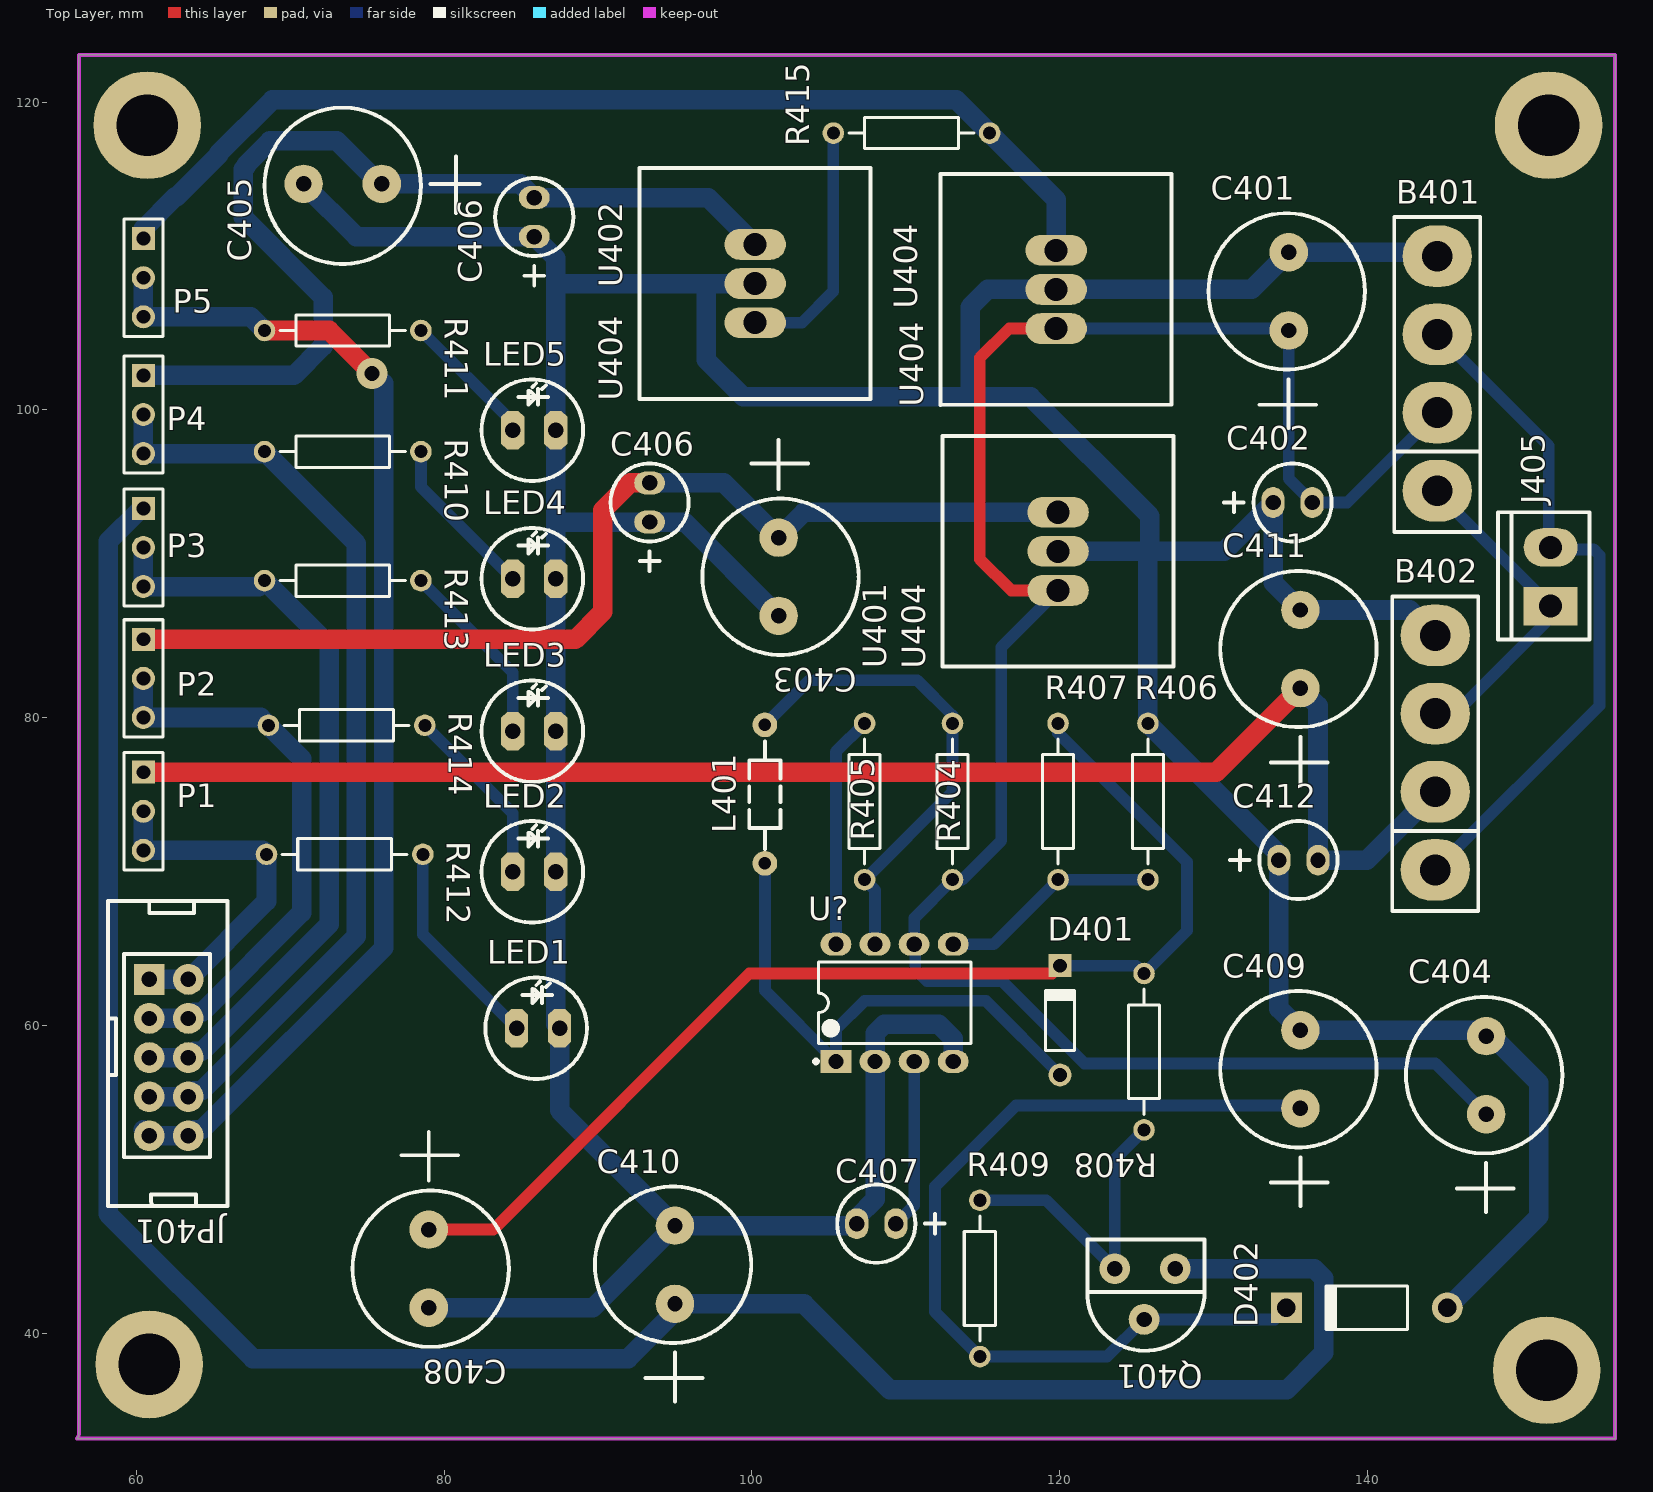
[diagram p0: Top Layer view]
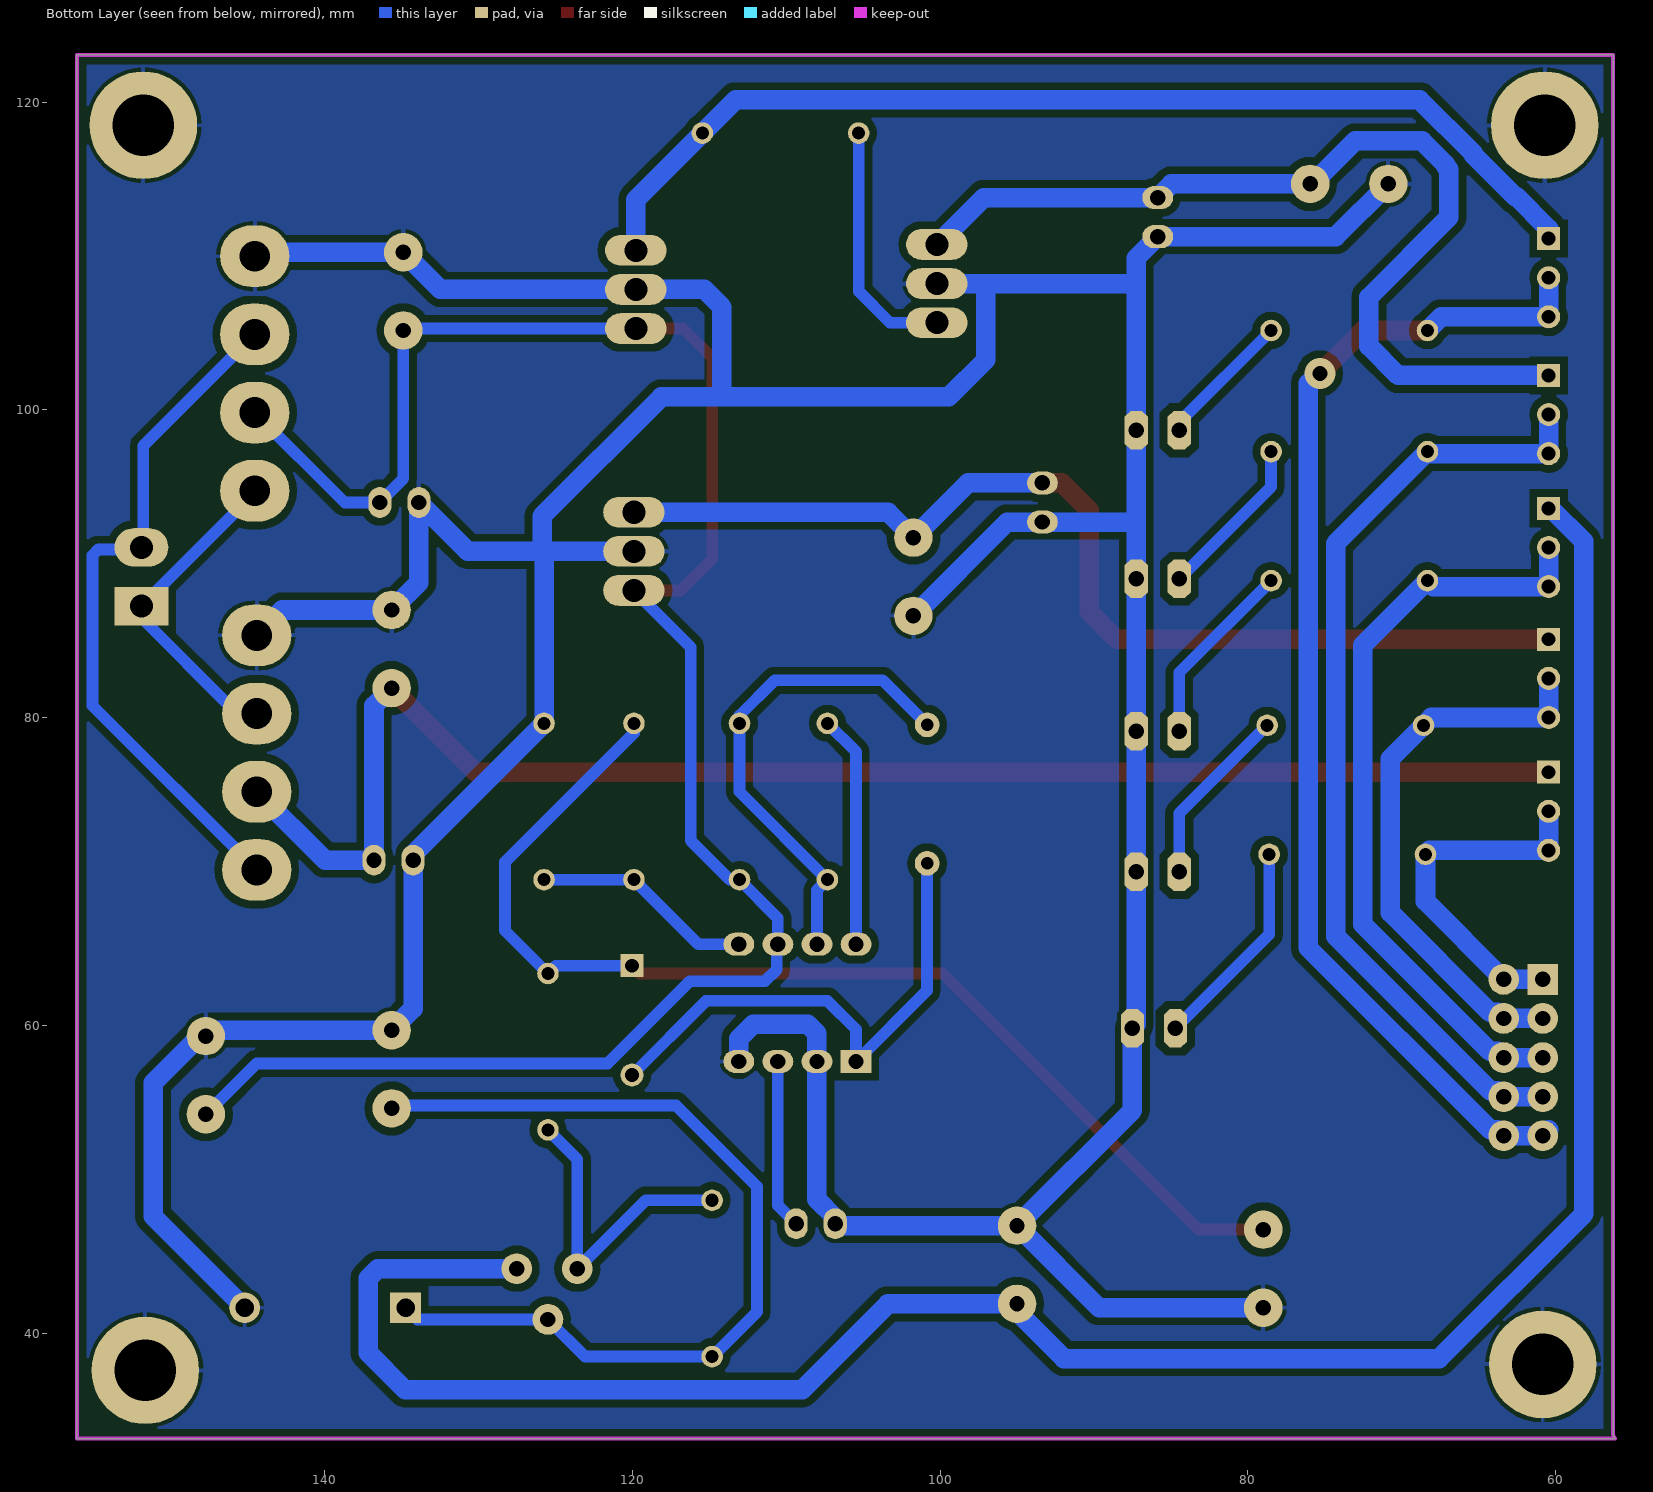
[diagram p1: Bottom Layer view, seen from below]
# Altium PCB MISC80623.PcbDoc
Units mm, origin at the board's own origin, x right, y up, seen from the top; angles counter-clockwise.
Board outline 99.95 x 89.92 mm, 2 copper layers (Top Layer, Bottom Layer); 47 components, 28 nets, 125 pads, 1 vias.

## Layer stack, top to bottom (the 12.6 mil dielectric is the usual default, probably not edited)
Top Solder: solder mask 0.0102, Solder Resist, Dk 3.5
Top Layer: signal copper 0.0356
Dielectric 1: dielectric 0.32, FR-4, Dk 4.8
Bottom Layer: signal copper 0.0356
Bottom Solder: solder mask 0.0102, Solder Resist, Dk 3.5

## Board outline
56.134,33.147 ccw(c55.827,33.454) 56.261,33.454 56.261,123.063 156.083,123.063 156.083,33.147

## Design rules (kind name [scope] priority, off if disabled: settings)
Clearance [All] p1: gap=0.508 ignorepadtopadclearanceinfootprint=FALSE except(0: Arc-Hole Track-Hole SMDPad-Hole THPad-Hole Via-Hole Fill-Hole Poly-Hole Region-Hole Text-Hole; 0.381: Via-Via)
PolygonConnect [All] p1: connectstyle=Relief reliefconductorwidth=0.254 reliefentries=4 polygonreliefangle="90 Angle" airgapwidth=0.254
RoutingVias [All] p1: holewidth=0.711 width=1.27 viastyle="Through Hole" minholewidth=0.711 minwidth=1.27 maxholewidth=0.711 maxwidth=1.27
SolderMaskExpansion [All] p1: expansion=0.102
Width [All] p1: maxlimit=1.27 minlimit=0.762 preferedwidth=0.762
30 further rules are at their usual default settings.

## Components (designator, comment, footprint, x,y, rotation, side; value= is the part's Value field where it differs from the comment)
B401 "Bridge1" B401 144.272,110.49 r90 top
B402 "Bridge1" B401 144.145,85.852 r90 top
C401 "1000UF/50V" C401 134.874,105.156 r90 top
C402 "104" DR 133.858,93.98 r0 top
C403 "47UF" C401 101.727,91.694 r270 top
C404 "100UF/50V" C401 147.701,54.229 r90 top
C405 "47UF" C401 75.946,114.681 r180 top
C406 "104" DR 85.852,111.252 r90 top
C406 "104" DR 93.345,92.71 r90 top
C407 "152" DR 109.347,47.117 r180 top
C408 "100UF/50V" C401 78.994,46.736 r270 top
C409 "100UF/50V" C401 135.636,54.61 r90 top
C410 "100UF/50V" C401 94.996,41.91 r90 top
C411 "1000UF/50V" C401 135.636,81.915 r90 top
C412 "104" DR 134.239,70.739 r0 top
D401 "4007" DO-35 120.015,60.331 r90 top
D402 "UPC574" DO-204AL 139.954,41.656 r180 top
J405 "AC18V" J405 151.892,87.249 r90 top
JP401 "POWER" JP401 60.833,62.992 r270 top
L401 "100UH/0.5W" AL0204 100.838,75.029 r90 top
LED1 "RED" LED 84.709,59.817 r0 top
LED2 "GREEN" LED 84.455,69.977 r0 top
LED3 "BLUE" LED 84.455,79.121 r0 top
LED4 "WHITE" LED 84.455,89.027 r0 top
LED5 "YELLOW" LED 84.455,98.679 r0 top
P1 "24V" HDR1X3 60.452,76.454 r270 top
P2 "LCD12V" HDR1X3 60.452,85.09 r270 top
P3 "33V" HDR1X3 60.452,93.599 r270 top
P4 "5V" HDR1X3 60.452,102.235 r270 top
P5 "IFA12V" HDR1X3 60.452,111.125 r270 top
Q401 "1815" Q401 127.508,44.196 r180 top
R404 "2.2/1W" AXIAL-0.4 113.03,74.549 r90 top
R405 "180" AXIAL-0.4 107.315,74.549 r90 top
R406 "1.5K" AXIAL-0.4 125.73,74.549 r90 top
R407 "39K" AXIAL-0.4 119.888,74.549 r90 top
R408 "47" AXIAL-0.4 125.476,58.293 r270 top
R409 "1.5K" AXIAL-0.4 114.808,43.561 r90 top
R410 "470" AXIAL-0.4 73.406,97.282 r0 top
R411 "680" AXIAL-0.4 73.406,105.156 r0 top
R412 "1K" AXIAL-0.4 73.533,71.12 r0 top
R413 "15K" AXIAL-0.4 73.406,88.9 r0 top
R414 "680" AXIAL-0.4 73.66,79.502 r0 top
R415 "18/0.5W" AXIAL-0.4 110.363,117.983 r180 top
U401 "7812" U404 119.888,90.805 r90 top
U402 "7805" U404 100.203,108.204 r90 top
U404 "7812" U404 119.761,107.823 r90 top
U? "MC34063" MC34063 108.966,61.468 r0 top

## Footprints (in the part's own frame and the unit in brackets; to place one, negate y for a bottom-side part, rotate by r counter-clockwise, add the part's x,y. Pads: shape width x height; smd on the part's side, far side on the other; paste and mask are expansions set on the pad)
AL0204 [mm] "9*2*4mm（脚距，直径，长度）"
  round 1.6 hole 0.8: 1(-4.5,0) 2(4.5,0)
  silkscreen extent -3.56,-1.02 3.43,1.02, body extent -4.75,-1.02 4.75,1.02, height 2.07
AXIAL-0.4 [mm] "Axial Device, Thru-Hole; 2 Leads; 0.4 in Pin Spacing"
  round 1.4 hole 0.85: 1(-5.08,0) 2(5.08,0)
  silkscreen extent -4.06,-1.02 4.06,1.02
B401 [mm]
  oval 4x4.5 hole 2: 1(-0.508,-0.254) 2(-5.588,-0.254) 3(-10.668,-0.254) 4(-15.748,-0.254)
  silkscreen extent -18.41,-3.05 2.03,2.54
C401 [mm]
  round 2.5 hole 1: 1(0,0) 2(5.08,0)
  silkscreen extent -6.35,-4.95 7.62,5.21
DO-35 [mm] "Diode, Axial; Body 3.8 x 1.9 mm (LxDia. max), Lead Dia. 0.53 mm (max)"
  round 1.5 hole 0.9: 1(-3.55,0)
  rect 1.5x1.5 hole 0.9: 2(3.55,0)
  silkscreen extent -1.95,-0.95 2.05,0.95
DO-204AL [mm] "Diode, Axial; Body 5.2 x 2.7 mm (LxDia. max), Lead Dia. 0.86 mm (max)"
  round 2 hole 1.2: 1(-5.23,0)
  rect 2x2 hole 1.2: 2(5.23,0)
  silkscreen extent -2.65,-1.4 2.75,1.4
DR [mm]
  oval 1.5x2 hole 1: 1(0,0) 2(2.54,0)
  silkscreen extent -3.17,-2.54 3.81,2.54
HDR1X3 [mm] "Connector; Header; 3 Position"
  rect 1.5x1.5 hole 0.9: 1(0,0)
  round 1.5 hole 0.9: 2(2.54,0) 3(5.08,0)
  silkscreen extent -1.27,-1.27 6.35,1.27
J405 [mm]
  rect 2.5x3.5 hole 1.5: 1(0,0)
  oval 2.5x3.5 hole 1.5: 2(3.81,0)
  silkscreen extent -2.16,-2.54 6.1,3.43
JP401 [mm]
  rect 2x2 hole 1: 1(0,0)
  round 2 hole 1: 2(0,2.54) 3(2.54,0) 4(2.54,2.54) 5(5.08,0) 6(5.08,2.54) 7(7.62,0) 8(7.62,2.54) 9(10.16,0) 10(10.16,2.54)
  silkscreen extent -5.08,-2.67 14.73,5.08
LED [mm]
  oct 1.5x2.5 hole 1: 1(0,0) 2(2.794,0)
  silkscreen extent -2.03,-3.3 4.57,3.3
MC34063 [mm]
  rect 2x1.5 hole 1 paste+0 mask+0.051: 1(-3.51,-3.81)
  oval 2x1.5 hole 1 paste+0 mask+0.051: 2(-0.97,-3.81) 3(1.57,-3.81) 4(4.11,-3.81) 5(4.11,3.81) 6(1.57,3.81) 7(-0.97,3.81) 8(-3.51,3.81)
  silkscreen extent -4.94,-3.93 5.26,2.65
Q401 [mm]
  round 2 hole 1: 1(0,0) 2(2.032,3.302) 3(3.937,0)
  silkscreen extent -1.91,-1.91 5.72,5.33
U404 [mm]
  oval 2x4 hole 1.5: 1(-2.54,0) 2(0,0) 3(2.54,0)
  silkscreen extent -7.5,-7.5 7.5,7.5

## Part data
B401 B402: "Full Wave Diode Bridge"
C401 C403 C404 C405 C408 C409 C410 C411: library part ELECTRO1
C402 C406 C406 C407 C412: library part CAP
D401: library part "Diode 1N4448", "High Conductance Fast Diode"
D402: library part "Diode 11DQ03", "Schottky Rectifier"
J405: library part "Header 2", "Header, 2-Pin"
JP401: library part "Header 5X2", "Header, 5-Pin, Dual row"
L401: library part INDUCTOR, "INDUCTOR"
LED1 LED2 LED3 LED4 LED5: library part LED0, "Typical INFRARED GaAs LED"
P1 P2 P3 P4 P5: library part "Header 3", "Header, 3-Pin"
Q401: library part 2N3904, "NPN General Purpose Amplifier"
R404 R405 R406 R407 R408 R409 R410 R411 R412 R413 R414 R415: library part Res2, "Resistor"
U401 U402 U404: library part AMS1117, "three-terminal voltage regulator"

## Free pads (board coordinates)
  round 7 hole 4: 0(60.833,37.973) 1(60.706,118.491) 2(151.765,118.491) 3(151.638,37.592)

## Via types
v1: diameter 2, hole 1, Top Layer to Bottom Layer, 1 vias

## Nets (pads, with @x,y where several pads share a name; then routed paths per layer and width w, separated by ;. In a path a pad name is that pad's centre, name@x,y a point inside that pad or via, vN(x,y) a via of type N, cw(c..) or ccw(c..) an arc to the next point about the centre after c; other vN are vias at no path point)
+5V: JP401.7 JP401.8 P4.2 P4.3 R410.1 | length 62.2
  Bottom Layer w1.27: P4.2 P4.3 68.199,97.155 R410.1 74.295,91.313 74.295,65.803 64.261,55.769 63.77,55.769 JP401.8 JP401.7
+5V-1: C405.1 C406.2@85.852,113.792 P4.1 U402.3 | length 63
  Bottom Layer w1.27: P4.1 70.231,102.235 72.136,104.14 72.136,107.315 66.929,112.522 66.929,115.633 67.127,115.831 67.127,115.921 68.681,117.475 73.025,117.475 75.819,114.681 C405.1 84.963,114.681 85.852,113.792 97.155,113.792 U402.3
+24V: JP401.1 JP401.2 P1.2 P1.3 R412.1 | length 23.4
  Bottom Layer w1.27: P1.2 P1.3 68.199,71.374 R412.1 68.453,68.072 JP401.2 JP401.1
+24V-1: B402.3 C411.1 C412.2 P1.1 | length 98.6
  Top Layer w1.27: P1.1 130.175,76.454 C411.1
  Bottom Layer w1.27: C411.1 136.779,80.772 C412.2 139.954,70.739 B402.3
+33V: JP401.5 JP401.6 P3.2 P3.3 R413.1 | length 49.9
  Bottom Layer w1.27: P3.2 P3.3 67.945,88.519 R413.1 72.517,84.709 72.517,66.565 64.261,58.309 63.77,58.309 JP401.6 JP401.5
+33V-1: C410.1 P3.1 Q401.1 | length 150.1
  Bottom Layer w1.27: P3.1 60.315,93.599 58.166,91.45 58.166,47.752 67.564,38.354 91.948,38.354 95.123,41.529 95.377,41.529 C410.1 103.378,41.91 108.966,36.322 134.747,36.322 137.16,38.735 137.16,43.561 136.525,44.196 Q401.1
GND: B401.1 B402.1 C401.2 C402.1 C403.2 C404.2 C405.2 C406.1 C407.2 C408.2 C409.2 C410.2 C411.2 C412.1 D402.1 LED1.2 LED2.2 LED3.2 LED4.2 LED5.2 pad.0 pad.1 pad.2 pad.3 R406.2 U401.2 U402.2 U404.2 U?.2 U?.4 | length 344.5
  Bottom Layer w1.27: C405.2 74.295,111.252 85.852,111.252 87.249,109.855 87.249,108.077 ; C408.2 89.662,41.656 C410.2 ; U402.2 97.028,108.204 ; C403.2 95.631,92.71 93.345,92.71 87.503,92.71 87.249,92.964 ; U?.4 113.076,59.136 112.141,60.071 108.585,60.071 107.996,59.482 U?.2 107.996,48.693 106.807,47.504 C407.2 106.68,46.99 C410.2 ; U401.2 125.857,90.805 ; B402.1 142.748,86.995 C411.2 133.858,88.773 C402.1 130.683,90.805 125.857,90.805 ; B401.1 144.272,110.236 C401.2 132.461,107.823 U404.2 115.316,107.823 114.173,106.68 114.173,100.965 114.046,100.838 ; D402.1 151.13,47.602 151.13,56.261 148.082,59.309 C404.2 147.32,59.69 C409.2 134.239,61.087 C412.1 134.239,71.12 R406.2 125.73,90.678 125.857,90.805 ; 87.249,92.964 LED5.2 87.249,108.077 ; 87.249,92.964 LED4.2 LED3.2 LED2.2 87.249,60.071 LED1.2 87.503,54.483 C410.2 ; 87.249,108.077 87.376,108.204 97.028,108.204 ; 97.028,108.204 97.028,103.251 99.441,100.838 114.046,100.838 ; 114.046,100.838 118.11,100.838 125.857,93.091 125.857,90.805
IFA12V: JP401.9 JP401.10 P5.2 P5.3 R411.1 | length 77.2
  Top Layer w1.27: R411.1 72.517,105.156 v1(75.311,102.362)
  Bottom Layer w1.27: JP401.9@60.436,53.229 JP401.9 JP401.10 63.77,53.229 64.261,53.229 76.073,65.041 76.073,101.727 v1@75.565,102.235 ; P5.2 P5.3 67.437,106.045 R411.1
IFA12V-1: P5.1 R415.1 U404.3 | length 69.5
  Bottom Layer w1.27: P5.1 60.452,111.76 62.54,113.848 62.629,113.848 65.349,116.568 65.349,116.657 68.834,120.142 113.284,120.142 R415.1 119.761,113.665 U404.3
LCD12V: JP401.3 JP401.4 P2.2 P2.3 R414.1 | length 36.7
  Bottom Layer w1.27: P2.2 P2.3 68.072,80.01 R414.1 70.739,77.343 70.739,67.327 64.261,60.849 63.77,60.849 JP401.4 JP401.3
LCD12V-1: C403.1 C406.2@93.345,95.25 P2.1 U401.3 | length 69.7
  Top Layer w1.27: P2.1 88.519,85.09 90.297,86.868 90.297,93.472 92.075,95.25 C406.2@93.345,95.25
  Bottom Layer w1.27: C406.2@93.345,95.25 98.171,95.25 C403.1 103.378,93.345 U401.3
NetB401_2: B401.2 B402.4 J405.2 | length 44.9
  Bottom Layer w0.762: B402.4 155.067,80.772 155.067,90.551 154.686,90.932 152.019,90.932 J405.2 ; B401.2 151.765,97.663 151.765,91.948 J405.2@152.273,91.44
NetB401_3: B401.3 C401.1 C402.2 C404.1 R404.1 U401.1 U404.1 U?.6 | length 132.2
  Top Layer w0.762: U404.1 116.713,105.283 114.808,103.378 114.808,90.297 116.84,88.265 U401.1
  Bottom Layer w0.762: U404.1 134.747,105.283 C401.1 134.874,95.532 136.398,94.008 C402.2 138.684,93.98 B401.3 ; U401.1 116.205,84.582 116.205,72.009 113.665,69.469 R404.1 110.536,66.975 U?.6 110.617,65.197 110.617,63.627 111.379,62.865 116.249,62.865 121.583,57.531 144.399,57.531 C404.1
NetB401_4: B401.4 B402.2 J405.1 | length 21.2
  Bottom Layer w0.762: B402.2 145.669,80.264 J405.1@152.273,86.868 ; B401.4 144.526,94.615 J405.1
NetC407_1: C407.1 U?.3 | length 11
  Bottom Layer w0.762: C407.1 110.536,48.306 U?.3
NetC408_1: C408.1 D401.2 R407.2 R408.1 | length 74.7
  Top Layer w0.762: C408.1 83.185,46.736 99.822,63.373 119.507,63.373 D401.2
  Bottom Layer w0.762: R407.2 119.888,78.994 128.27,70.612 128.27,66.167 R408.1 124.968,63.881 D401.2
NetC409_1: C409.1 D402.2 Q401.2 R409.1 | length 59.6
  Bottom Layer w0.762: D402.2 133.962,40.894 Q401.2 123.063,38.481 R409.1 111.887,41.402 111.887,49.53 117.159,54.802 135.636,54.802 C409.1
NetD401_1: D401.1 L401.1 U?.1 | length 34.2
  Bottom Layer w0.762: L401.1 100.838,62.276 U?.1 105.456,59.736 107.315,61.595 115.201,61.595 D401.1
NetL401_2: L401.2 R404.2 R405.1 U?.7 | length 31.8
  Bottom Layer w0.762: L401.2 103.732,82.423 110.744,82.423 113.03,80.137 R404.2 113.03,75.184 R405.1 107.996,68.788 U?.7
NetLED1_1: LED1.1 R412.2 | length 13.8
  Bottom Layer w0.762: R412.2 78.613,65.913 LED1.1
NetLED2_1: LED2.1 R414.2 | length 11.9
  Bottom Layer w0.762: R414.2 84.455,73.787 LED2.1
NetLED3_1: LED3.1 R413.2 | length 12.3
  Bottom Layer w0.762: R413.2 84.455,82.931 LED3.1
NetLED4_1: LED4.1 R410.2 | length 10.7
  Bottom Layer w0.762: R410.2 78.486,94.996 LED4.1
NetLED5_1: LED5.1 R411.2 | length 8.9
  Bottom Layer w0.762: R411.2 84.455,99.187 LED5.1
NetQ401_3: Q401.3 R408.2 R409.2 | length 20.4
  Bottom Layer w0.762: R409.2 119.126,48.641 Q401.3 123.571,51.308 R408.2
NetR405_2: R405.2 U?.8 | length 15.1
  Bottom Layer w0.762: U?.8 105.456,77.77 R405.2
NetR406_1: R406.1 R407.1 U?.5 | length 14.4
  Bottom Layer w0.762: U?.5 115.697,65.278 R407.1 R406.1
NetR415_2: R415.2 U402.1 | length 16.2
  Bottom Layer w0.762: U402.1 103.251,105.664 105.283,107.696 R415.2

## Polygon pours and split planes (outlines as drawn)
GND on Bottom Layer "Top Layer-No Net" (solid, remove dead copper, pour order 4): 50.673,127.381 51.181,127.889 161.29,127.889 161.29,28.575 162.56,27.305 51.054,27.305

## Keep-outs
Keep-Out Layer:
  lines w0.254: 56.134,33.147 ccw(c55.827,33.454) 56.261,33.454 56.261,123.063 57.404,123.063 156.083,123.063 156.083,33.147 56.134,33.147